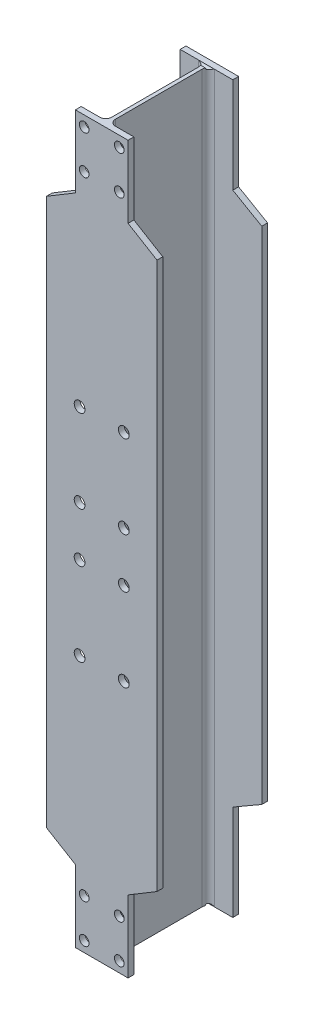
SolidWorks part; units mm, degrees
material "Q235B"
ref_plane "Front Plane" through (0, 0, 0) normal (0, 0, 1) x (1, 0, 0)
ref_plane "Top Plane" through (0, 0, 0) normal (0, 1, 0) x (1, 0, 0)
ref_plane "Right Plane" through (0, 0, 0) normal (1, 0, 0) x (0, 0, -1)
sketch "Sketch1" plane through (0, 0, 0) normal (0, 1, 0) x (1, 0, 0)
  line L0 (-450.3232, 0) -> (248.6177, 0) construction
  line L1 (0, 298.6096) -> (0, -328.4825) construction
  line L2 (-6.5, -157) -> (-6.5, 157)
  line L3 (-28.5, 179) -> (-200, 179)
  line L4 (-200, 179) -> (-200, 200)
  line L5 (-200, 200) -> (200, 200)
  line L6 (6.5, -157) -> (6.5, 157)
  line L7 (200, 179) -> (200, 200)
  line L8 (28.5, 179) -> (200, 179)
  line L9 (28.5, -179) -> (200, -179)
  line L10 (200, -179) -> (200, -200)
  line L11 (-200, -200) -> (200, -200)
  line L12 (-200, -179) -> (-200, -200)
  line L13 (-28.5, -179) -> (-200, -179)
  arc A0 (-6.5, 157) -> (-28.5, 179) centre (-28.5, 157) ccw
  arc A1 (28.5, 179) -> (6.5, 157) centre (28.5, 157) ccw
  arc A2 (-6.5, -157) -> (-28.5, -179) centre (-28.5, -157) cw
  arc A3 (6.5, -157) -> (28.5, -179) centre (28.5, -157) ccw
  point P5 (0, -200)
  point P14 (0, 200)
  point P17 (6.5, 0)
  point P20 (-6.5, 0)
  dimension "D5" = 22
  dimension "D1" = 400
  dimension "D2" = 400
  dimension "D3" = 21
  dimension "D4" = 13
extrude "Extrude1" add sketch "Sketch1" along normal mid plane 2625
sketch "Sketch3" plane through (0, 0, 200) normal (0, 0, 1) x (1, 0, 0)
  line L0 (0, 1903.1694) -> (0, -1746.7445) construction
  line L1 (-656.1155, 0) -> (690.8766, 0) construction
  line L2 (-95.25, 1312.5) -> (-95.25, 1052.15)
  line L3 (-200, 1312.5) -> (200, 1312.5) construction
  line L4 (-95.25, 1052.15) -> (-200, 989.2099)
  line L5 (-200, 1312.5) -> (-200, -1312.5) construction
  line L6 (-200, 989.2099) -> (-200, 1312.5)
  line L7 (-200, 1312.5) -> (-95.25, 1312.5)
  line L8 (95.25, 1052.15) -> (200, 989.2099)
  line L9 (95.25, 1312.5) -> (95.25, 1052.15)
  line L10 (200, 1312.5) -> (95.25, 1312.5)
  line L11 (200, 989.2099) -> (200, 1312.5)
  line L12 (200, -989.2099) -> (200, -1312.5)
  line L13 (200, -1312.5) -> (95.25, -1312.5)
  line L14 (95.25, -1312.5) -> (95.25, -1052.15)
  line L15 (95.25, -1052.15) -> (200, -989.2099)
  line L16 (-200, -1312.5) -> (-95.25, -1312.5)
  line L17 (-200, -989.2099) -> (-200, -1312.5)
  line L18 (-95.25, -1052.15) -> (-200, -989.2099)
  line L19 (-95.25, -1312.5) -> (-95.25, -1052.15)
  dimension "D1" = 260.35
  dimension "D2" = 59
  dimension "D3" = 190.5
extrude "Cut-Extrude2" cut sketch "Sketch3" against normal blind 30
sketch "Sketch5" plane through (0, 0, -200) normal (0, 0, -1) x (-1, 0, 0)
  line L0 (-517.8475, 0) -> (669.6019, 0) construction
  line L1 (-200, 1312.5) -> (-95.25, 1312.5)
  line L2 (-95.25, 1312.5) -> (-95.25, 966.425)
  line L3 (-95.25, 966.425) -> (-200, 905.9476)
  line L4 (-200, 1312.5) -> (-200, -1312.5) construction
  line L5 (-200, 905.9476) -> (-200, 1312.5)
  line L7 (0, 0) -> (0, 1492.5764) construction
  line L8 (200, 905.9476) -> (200, 1312.5)
  line L9 (95.25, 966.425) -> (200, 905.9476)
  line L10 (95.25, 1312.5) -> (95.25, 966.425)
  line L11 (200, 1312.5) -> (95.25, 1312.5)
  line L12 (200, -1312.5) -> (95.25, -1312.5)
  line L13 (95.25, -1312.5) -> (95.25, -966.425)
  line L14 (95.25, -966.425) -> (200, -905.9476)
  line L15 (200, -905.9476) -> (200, -1312.5)
  line L16 (-200, -905.9476) -> (-200, -1312.5)
  line L17 (-95.25, -966.425) -> (-200, -905.9476)
  line L18 (-95.25, -1312.5) -> (-95.25, -966.425)
  line L19 (-200, -1312.5) -> (-95.25, -1312.5)
  dimension "D1" = 346.075
  dimension "D2" = 120
extrude "Cut-Extrude3" cut sketch "Sketch5" against normal blind 30
sketch "Sketch2" plane through (0, 0, 200) normal (0, 0, 1) x (1, 0, 0)
  line L0 (0, 1318.0242) -> (0, -1324.501) construction
  line L1 (-454.6588, 0) -> (423.8024, 0) construction
  line L2 (-95.25, 1312.5) -> (95.25, 1312.5) construction
  circle A0 centre (-80, 390) radius 19.5
  circle A1 centre (80, 390) radius 19.5
  circle A2 centre (80, -390) radius 19.5
  circle A3 centre (-80, -390) radius 19.5
  circle A4 centre (63.5, 1274.5) radius 17.5
  circle A5 centre (63.5, 1134.5) radius 17.5
  circle A6 centre (-63.5, 1274.5) radius 17.5
  circle A7 centre (-63.5, 1134.5) radius 17.5
  circle A8 centre (63.5, -1134.5) radius 17.5
  circle A9 centre (-63.5, -1134.5) radius 17.5
  circle A10 centre (63.5, -1274.5) radius 17.5
  circle A11 centre (-63.5, -1274.5) radius 17.5
  circle A12 centre (-80, 90) radius 19.5
  circle A13 centre (80, 90) radius 19.5
  circle A14 centre (-80, -90) radius 19.5
  circle A15 centre (80, -90) radius 19.5
  dimension "D1" = 780
  dimension "D2" = 160
  dimension "D3" = 39
  dimension "D4" = 140
  dimension "D5" = 127
  dimension "D6" = 35
  dimension "D7" = 38
  dimension "D8" = 2
  dimension "D9" = 2
extrude "Cut-Extrude1" cut sketch "Sketch2" against normal blind 50.8
sketch "Sketch6" plane through (0, 0, 0) normal (1, 0, 0) x (0, 0, -1)
  line L0 (179, 1312.5) -> (157, 1312.5) construction
  line L1 (179, 1312.5) -> (179, -1312.5) construction
  line L2 (0, 0) -> (790.9339, 0) construction
  circle A0 centre (172.65, 1312.5) radius 6.35
  circle A1 centre (172.65, -1312.5) radius 6.35
  dimension "D1" = 12.7
extrude "Cut-Extrude4" cut sketch "Sketch6" against normal mid plane 60
